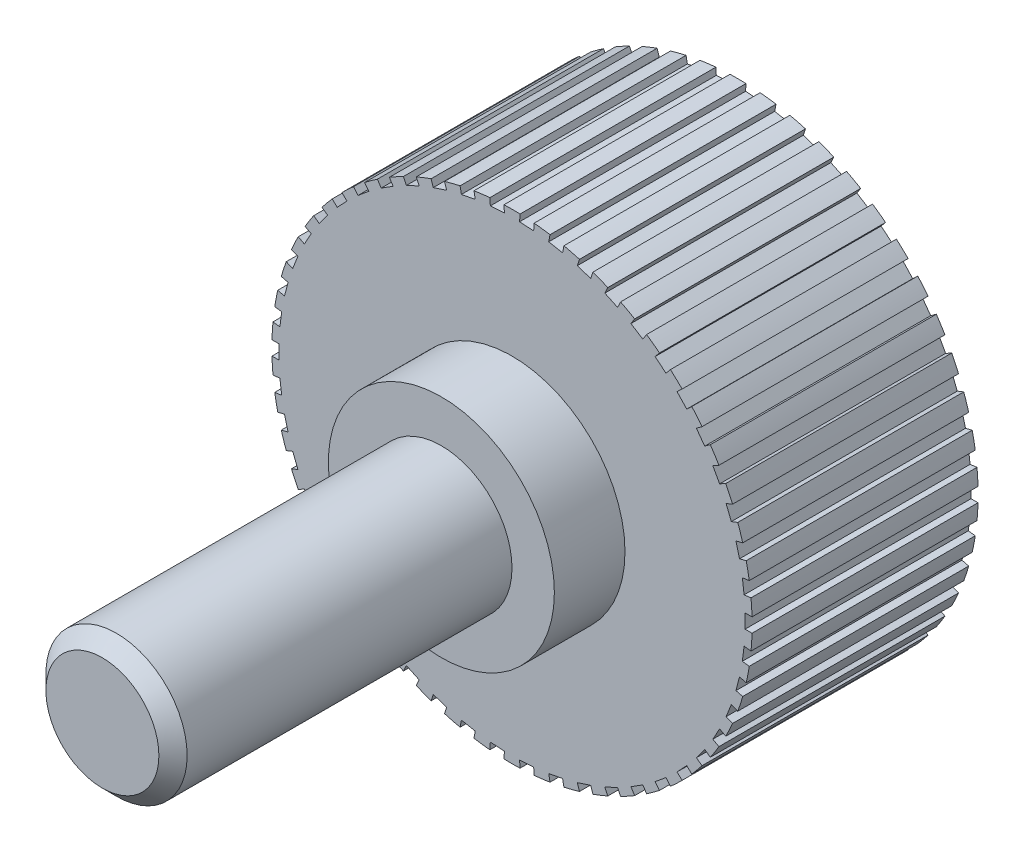
from build123d import *

# Parameters (mm, degrees)
SKETCH1_R           = 8.5
BOSS_EXTRUDE1_DEPTH = 8
SKETCH2_R           = 4
BOSS_EXTRUDE2_DEPTH = 2.5
SKETCH3_R           = 2.5
BOSS_EXTRUDE3_DEPTH = 12
CHAMFER1_SIZE       = 0.5
SKETCH5_W           = 0.5
SKETCH5_H           = 0.5
CUT_EXTRUDE2_DEPTH  = 10
CIRPATTERN2_COUNT   = 50


with BuildPart() as part:
    # Sketch1 → Boss-Extrude1 (new body)
    with BuildSketch(Plane.XY):
        Circle(SKETCH1_R)
    extrude(amount=BOSS_EXTRUDE1_DEPTH)

    # Sketch2 → Boss-Extrude2 (add)
    with BuildSketch(Plane.XY.offset(8)):
        Circle(SKETCH2_R)
    extrude(amount=BOSS_EXTRUDE2_DEPTH)

    # Sketch3 → Boss-Extrude3 (add)
    with BuildSketch(Plane.XY.offset(10.5)):
        Circle(SKETCH3_R)
    extrude(amount=BOSS_EXTRUDE3_DEPTH)

    # Chamfer1
    chamfer1_edges = [part.edges().sort_by_distance(p)[0] for p in [
        (-2.5, 0, 22.5),
    ]]
    chamfer(chamfer1_edges, length=CHAMFER1_SIZE)

    # Sketch5 → Cut-Extrude2 (cut)
    with BuildSketch(Plane.XY.offset(8)):
        with Locations((8.5, 0)):
            Rectangle(SKETCH5_W, SKETCH5_H)
    cut_extrude2 = extrude(amount=-CUT_EXTRUDE2_DEPTH, mode=Mode.SUBTRACT)

    # CirPattern2: Cut-Extrude2 ×50 about axis
    cirpattern2_axis = Axis((0, 0, 0), (0, 0, 1))
    for i in range(1, CIRPATTERN2_COUNT):
        add(cut_extrude2.rotate(cirpattern2_axis, i * 360 / CIRPATTERN2_COUNT), mode=Mode.SUBTRACT)


solid = part.part
